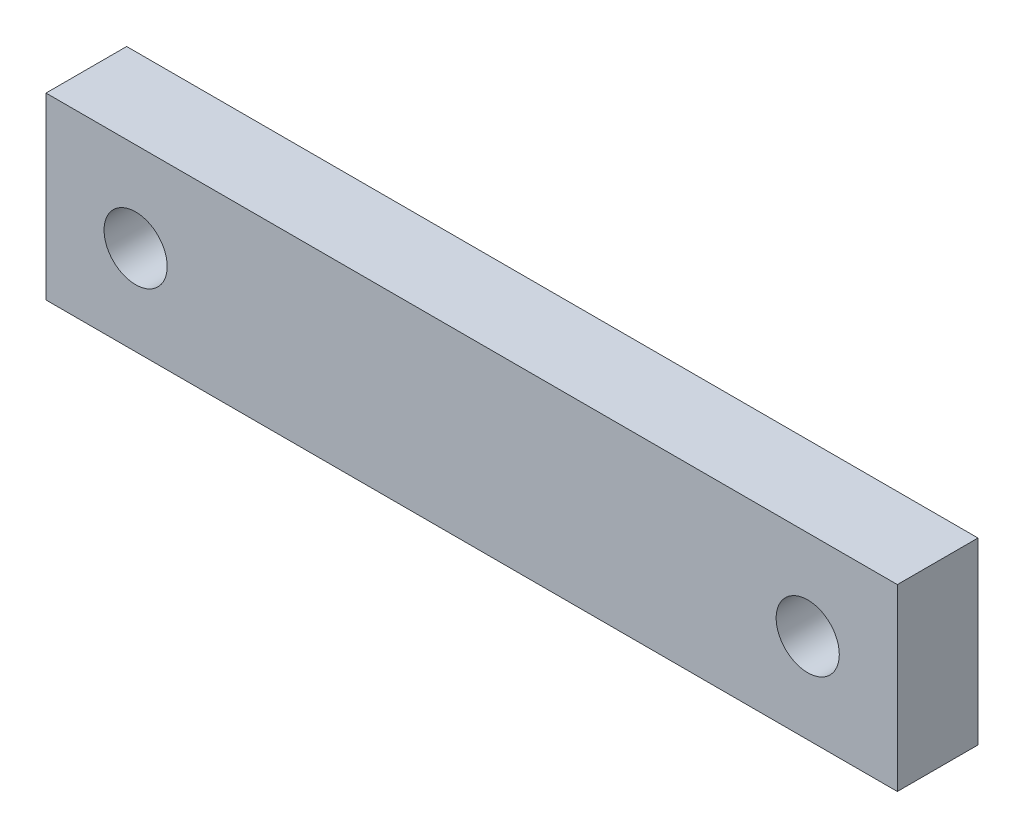
from build123d import *

# Parameters (mm, degrees)
SKETCH1_W                = 380
SKETCH1_H                = 80
BOSS_EXTRUDE1_DEPTH      = 18
F_1_1_4_7_TAPPED_HOLE1_D = 28.17876


with BuildPart() as part:
    # Sketch1 → Boss-Extrude1 (new, symmetric)
    with BuildSketch(Plane.XY):
        Rectangle(SKETCH1_W, SKETCH1_H)
    extrude(amount=BOSS_EXTRUDE1_DEPTH, both=True)

    # 1-1/4-7 Tapped Hole1 (through all)
    with Locations(Plane.XY.offset(18)):
        with Locations((-150, 0), (150, 0)):
            Hole(F_1_1_4_7_TAPPED_HOLE1_D / 2)


solid = part.part
